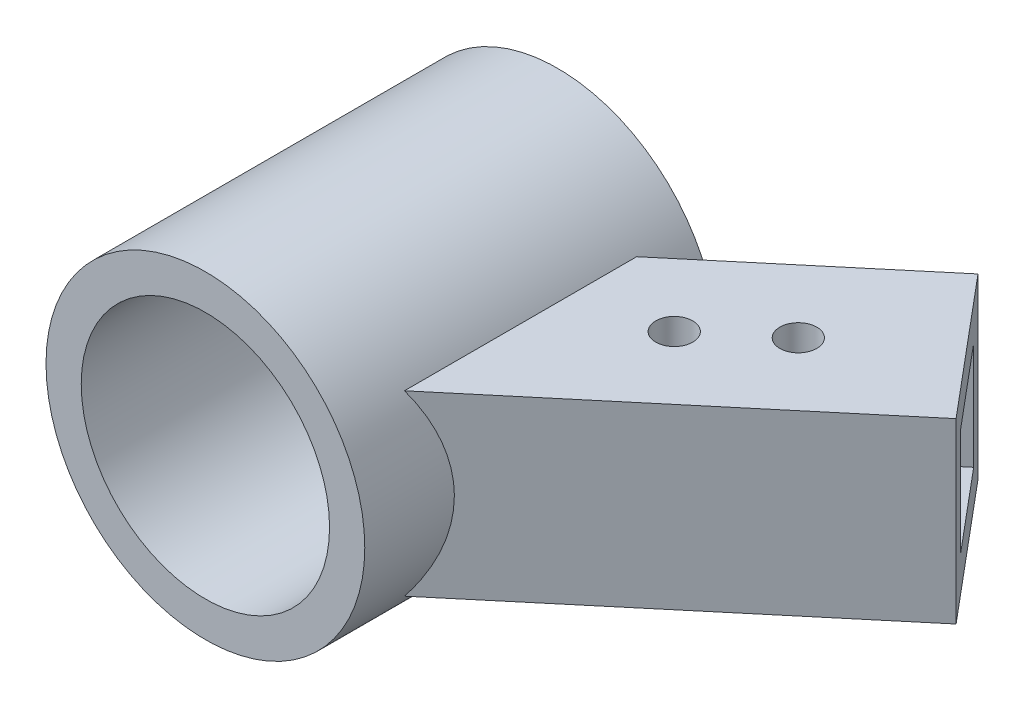
SolidWorks part; units mm, degrees
ref_plane "前视基准面" through (0, 0, 0) normal (0, 0, 1) x (1, 0, 0)
ref_plane "上视基准面" through (0, 0, 0) normal (0, 1, 0) x (1, 0, 0)
ref_plane "右视基准面" through (0, 0, 0) normal (1, 0, 0) x (0, 0, -1)
sketch "草图1" plane through (0, 0, 0) normal (0, 0, 1) x (1, 0, 0)
  circle A0 centre (0, 0) radius 35.25
  circle A1 centre (0, 0) radius 45.25
  dimension "D1" = 70.5
  dimension "D2" = 10
extrude "凸台-拉伸1" add sketch "草图1" along normal mid plane 100
sketch "草图2" plane through (0, 0, 0) normal (0, 1, 0) x (1, 0, 0)
  line L0 (45.25, 41.3525) -> (90.238, 79.1019)
  line L1 (35.25, -32.9615) -> (122.6987, 40.4167)
  line L2 (77.7108, 2.6673) -> (122.6987, 40.4167) construction
  line L3 (35.25, 19.9075) -> (96.6658, 71.4415)
  line L4 (35.25, -19.9075) -> (116.2709, 48.0771)
  line L5 (45.25, -50) -> (45.25, 50) construction
  line L6 (72.7027, 11.5191) -> (116.2709, 48.0771) construction
  line L7 (79.1305, 3.8586) -> (122.6987, 40.4167) construction
  line L8 (51.6779, 33.6921) -> (96.6658, 71.4415) construction
  line L10 (45.25, -50) -> (45.25, 50) construction
  line L11 (35.25, 32.9615) -> (35.25, -32.9615)
  line L12 (90.238, 79.1019) -> (122.6987, 40.4167)
  line L15 (45.25, 41.3525) -> (35.25, 32.9615)
  line L16 (0, 0) -> (35.25, 0) construction
  dimension "D1" = 30.5
  dimension "D4" = 130
  dimension "D5" = 10
  dimension "D6" = 120
  dimension "D2" = 10
  dimension "D3" = 10
extrude "凸台-拉伸2" add sketch "草图2" along normal mid plane 30.5
sketch "草图4" plane through (0, 15.25, 0) normal (0, 1, 0) x (1, 0, 0)
  line L0 (90.238, 79.1019) -> (122.6987, 40.4167)
  line L1 (122.6987, 40.4167) -> (35.25, -32.9615)
  line L3 (35.25, 32.9615) -> (90.238, 79.1019)
  line L4 (35.25, 32.9615) -> (35.25, -32.9615)
  line L7 (45.25, -11.5165) -> (45.25, 28.2985) construction
  dimension "D1" = 10
extrude "凸台-拉伸3" add sketch "草图4" along normal blind 10
mirror "镜向1" about plane through (0, 0, 0) normal (0, 1, 0) of "凸台-拉伸3"
sketch "草图5" plane through (0, 25.25, 0) normal (0, 1, 0) x (1, 0, 0)
  line L0 (106.4683, 59.7593) -> (80.4228, 37.9045) construction
  line L1 (122.6987, 40.4167) -> (90.238, 79.1019) construction
  line L2 (80.4228, 37.9045) -> (61.2717, 21.8348) construction
  circle A0 centre (80.4228, 37.9045) radius 5.25
  circle A1 centre (61.2717, 21.8348) radius 5.25
  dimension "D3" = 10.5
  dimension "D1" = 34
  dimension "D2" = 25
extrude "切除-拉伸1" cut sketch "草图5" against normal mid plane 165
